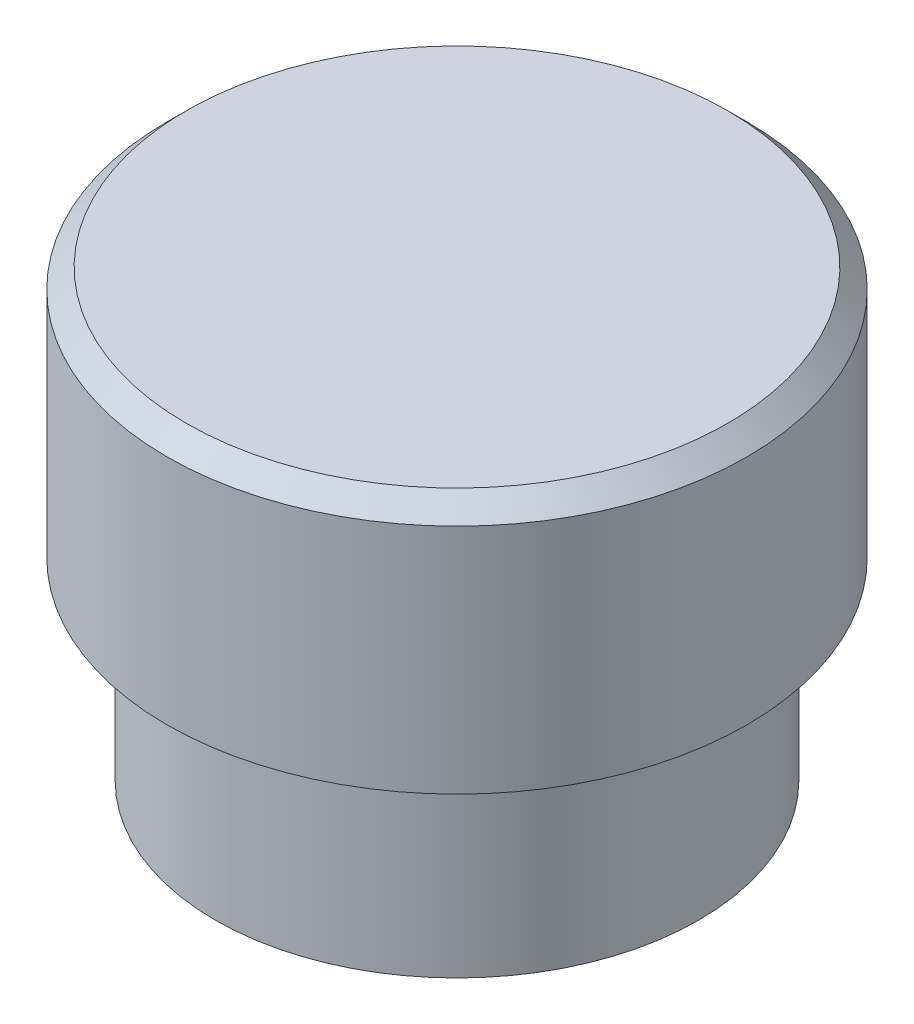
SolidWorks part; units mm, degrees
ref_plane "前视基准面" through (0, 0, 0) normal (0, 0, 1) x (1, 0, 0)
ref_plane "上视基准面" through (0, 0, 0) normal (0, 1, 0) x (1, 0, 0)
ref_plane "右视基准面" through (0, 0, 0) normal (1, 0, 0) x (0, 0, -1)
sketch "草图1" plane through (0, 0, 0) normal (0, 1, 0) x (1, 0, 0)
  circle A0 centre (0, 0) radius 15
  dimension "D1" = 30
extrude "凸台-拉伸1" add sketch "草图1" along normal blind 13
sketch "草图2" plane through (0, 0, 0) normal (0, -1, 0) x (1, 0, 0)
  circle A0 centre (0, 0) radius 12.5
  dimension "D1" = 25
extrude "凸台-拉伸2" add sketch "草图2" along normal blind 10
chamfer "倒角1" distance 1 angle 45 1 edges at (0, 13, 15)
